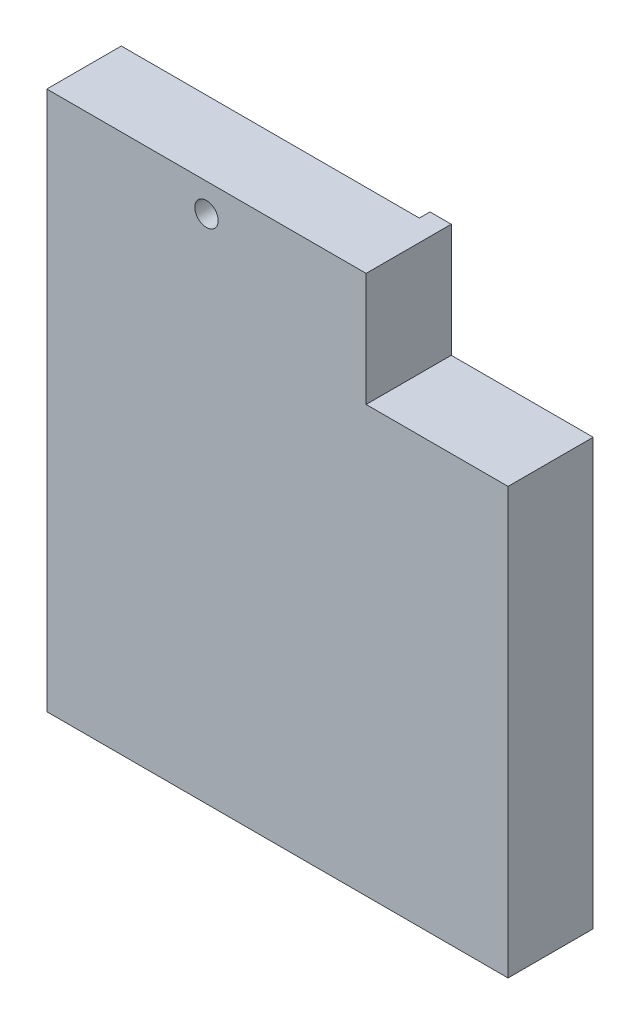
SolidWorks part; units mm, degrees
ref_plane "前视基准面" through (0, 0, 0) normal (0, 0, 1) x (1, 0, 0)
ref_plane "上视基准面" through (0, 0, 0) normal (0, 1, 0) x (1, 0, 0)
ref_plane "右视基准面" through (0, 0, 0) normal (1, 0, 0) x (0, 0, -1)
sketch "草图1" plane through (0, 0, 0) normal (0, 0, 1) x (1, 0, 0)
  line L1 (-32.5, -30) -> (32.5, -30)
  line L2 (-32.5, -30) -> (-32.5, 30)
  line L3 (-32.5, 30) -> (32.5, 30)
  line L4 (32.5, -30) -> (32.5, 30)
  line L5 (-32.5, -30) -> (32.5, 30) construction
  line L6 (-32.5, 30) -> (32.5, -30) construction
  point P0 (0, 0)
  dimension "D1" = 60
  dimension "D2" = 65
extrude "凸台-拉伸1" add sketch "草图1" along normal blind 12
sketch "草图4" plane through (0, 0, 0) normal (0, 0, -1) x (-1, 0, 0)
  line L0 (-12.5, 30) -> (-12.5, 46)
  line L2 (-12.5, 46) -> (32.5, 46)
  line L3 (32.5, 46) -> (32.5, 30)
  line L4 (32.5, 30) -> (-12.5, 30)
  point P2 (0, 0)
  point P3 (32.5, 30)
  point P4 (0, 0)
  dimension "D1" = 16
  dimension "D2" = 45
extrude "凸台-拉伸2" add sketch "草图4" against normal up to surface (12 mm away) up to face at (0, 0, 12)
sketch "草图5" plane through (0, 0, 0) normal (0, 0, -1) x (-1, 0, 0)
  line L0 (32.5, -30) -> (-32.5, -30) construction
  line L1 (32.5, 46) -> (-9.5, 46)
  line L2 (32.5, 46) -> (32.5, -30)
  line L3 (32.5, -30) -> (-9.5, -30)
  line L4 (-9.5, 46) -> (-9.5, -30)
  dimension "D1" = 42
extrude "切除-拉伸1" cut sketch "草图5" against normal blind 1.5
hole_wizard "M4 螺纹孔1" positions "3D草图1" profile "草图6" tap size "M4" standard "GB" end condition up to next
sketch3d "3D草图1"
  line L0 (-10, 46, 12) -> (-10, 42, 12)
  line L1 (12.5, 46, 12) -> (-32.5, 46, 12) construction
  point P0 (-10, 42, 12)
  dimension "D1" = 4
sketch "草图6" plane through (-10, 42, 12) normal (1, 0, 0) x (0, -1, 0)
  line L0 (0, 0) -> (0, 10.5)
  line L1 (0, 10.5) -> (1.65, 10.5)
  line L2 (1.65, 10.5) -> (1.65, 0)
  line L5 (1.65, 0) -> (0, 0)
  line L11 (0, -6.35) -> (0, 107.95) construction
  dimension "通孔螺纹孔钻头直径" = 3.3
  dimension "通孔螺纹孔钻头深度" = 10.5
cosmetic thread "孔螺蚊线1" parameters "D2"=4
